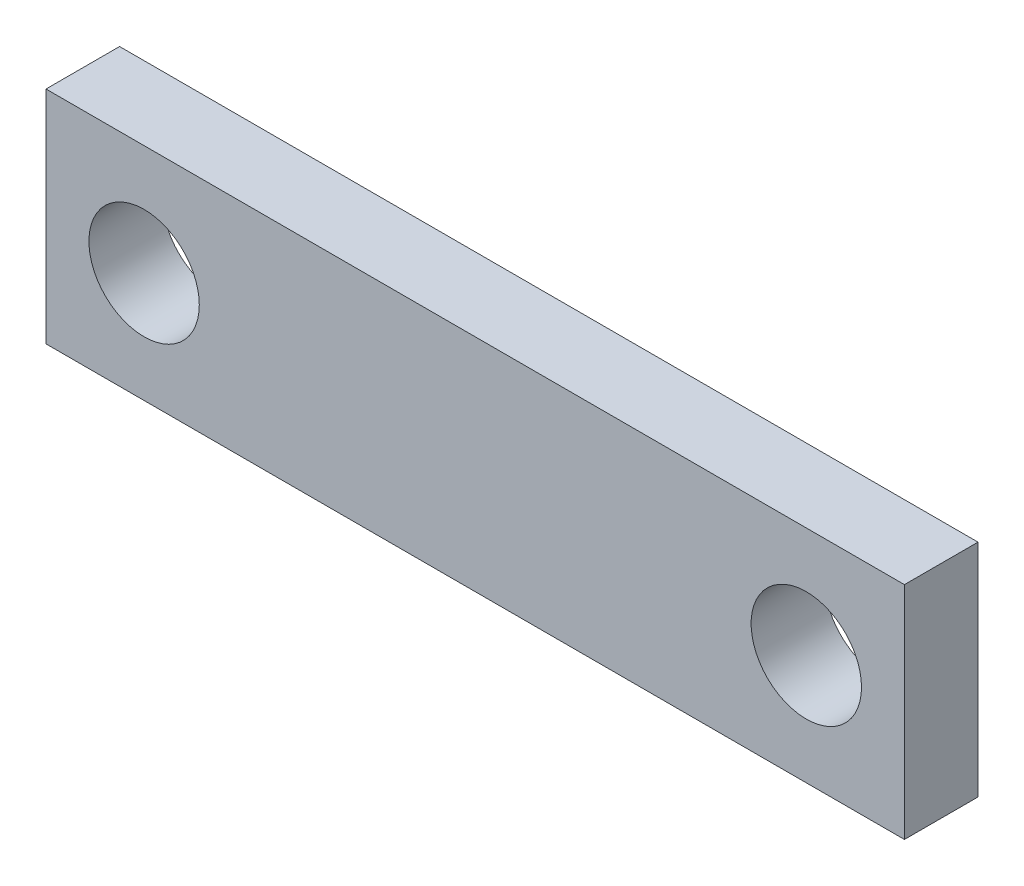
from build123d import *

# Parameters (mm, degrees)
SKETCH_1_W      = 35
SKETCH_1_H      = 9
SKETCH_1_R      = 2.25
EXTRUDE_1_DEPTH = 1.5


with BuildPart() as part:
    # 草图1 → 凸台-拉伸1 (new, symmetric)
    with BuildSketch(Plane.XY):
        Rectangle(SKETCH_1_W, SKETCH_1_H)
        with Locations((-13.5, 0)):
            Circle(SKETCH_1_R, mode=Mode.SUBTRACT)
        with Locations((13.5, 0)):
            Circle(SKETCH_1_R, mode=Mode.SUBTRACT)
    extrude(amount=EXTRUDE_1_DEPTH, both=True)


solid = part.part
